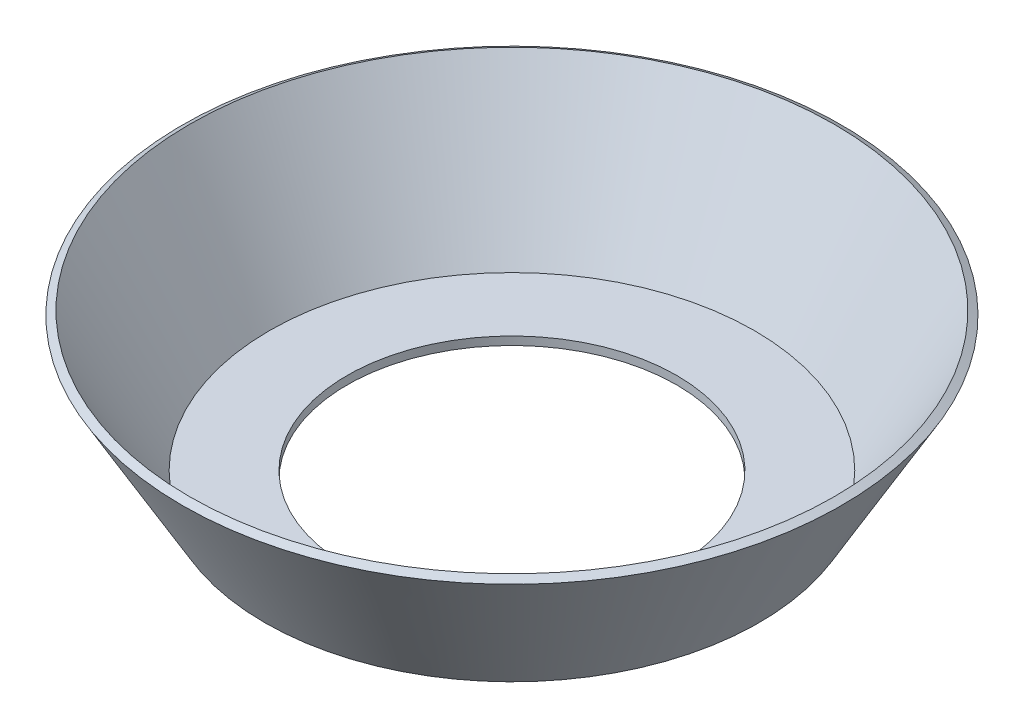
from build123d import *


with BuildPart() as part:
    # Sketch1 → Revolve1 (revolve)
    with BuildSketch(Plane.XY, mode=Mode.PRIVATE) as revolve1_sk:
        Polygon((10, 0), (15, 0), (20, 8.660254038), (19.566987298, 8.910254038), (14.711324865, 0.5), (10, 0.5), align=None)
    revolve(revolve1_sk.sketch.rotate(Axis((0, 20.263157895, 0), (0, -1, 0)), 90), axis=Axis((0, 20.263157895, 0), (0, -1, 0)))


solid = part.part
